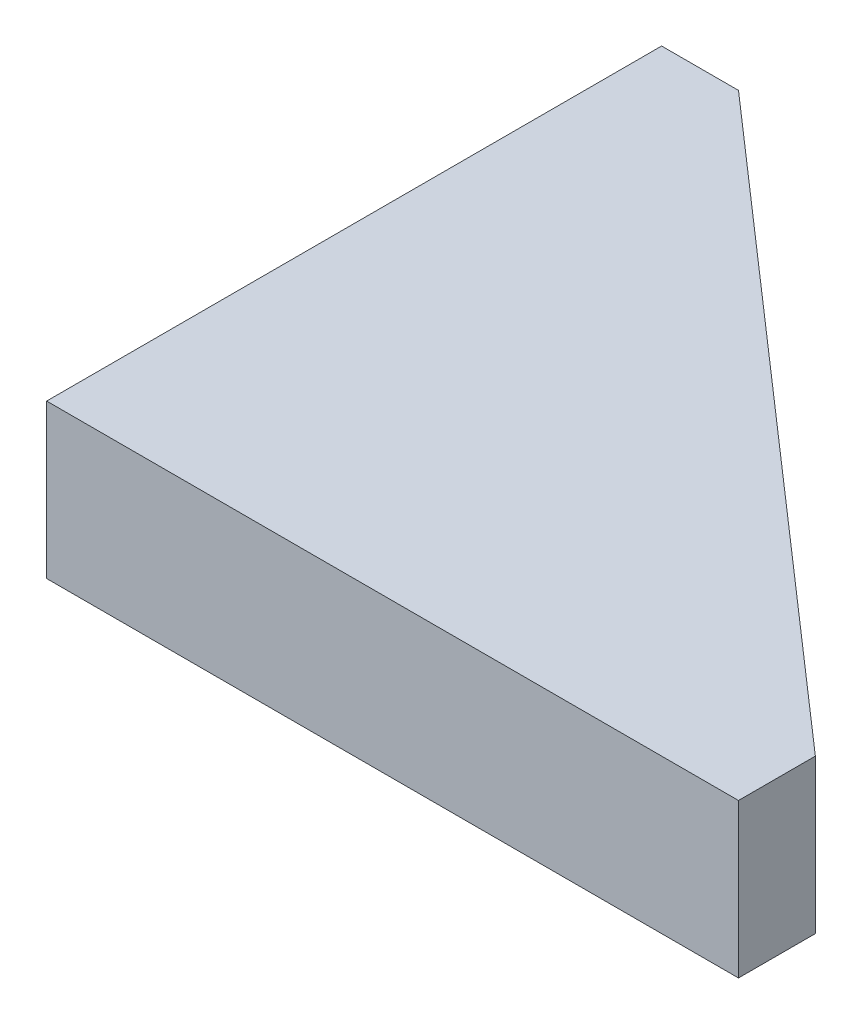
SolidWorks part; units mm, degrees
ref_plane "前视基准面" through (0, 0, 0) normal (0, 0, 1) x (1, 0, 0)
ref_plane "上视基准面" through (0, 0, 0) normal (0, 1, 0) x (1, 0, 0)
ref_plane "右视基准面" through (0, 0, 0) normal (1, 0, 0) x (0, 0, -1)
sketch "草图1" plane through (0, 0, 0) normal (0, 1, 0) x (1, 0, 0)
  line L1 (-22.5, 20) -> (22.5, 20)
  line L2 (-22.5, 20) -> (-22.5, -20)
  line L3 (-22.5, -20) -> (22.5, -20)
  line L4 (22.5, 20) -> (22.5, -20)
  line L5 (-22.5, 20) -> (22.5, -20) construction
  line L6 (-22.5, -20) -> (22.5, 20) construction
  point P0 (0, 0)
  dimension "D1" = 45
  dimension "D2" = 40
extrude "凸台-拉伸1" add sketch "草图1" along normal blind 10
sketch "草图2" plane through (0, 10, 0) normal (0, 1, 0) x (1, 0, 0)
  line L0 (22.5, 20) -> (-17.5, 20)
  line L1 (22.5, 20) -> (-22.5, 20) construction
  line L2 (-17.5, 20) -> (22.5, -15)
  line L3 (22.5, -20) -> (22.5, 20) construction
  line L4 (22.5, -15) -> (22.5, 20)
  line L5 (-22.5, 20) -> (-22.5, -20) construction
  line L6 (-22.5, -20) -> (22.5, -20) construction
  dimension "D1" = 5
  dimension "D2" = 5
extrude "切除-拉伸1" cut sketch "草图2" against normal blind 20
